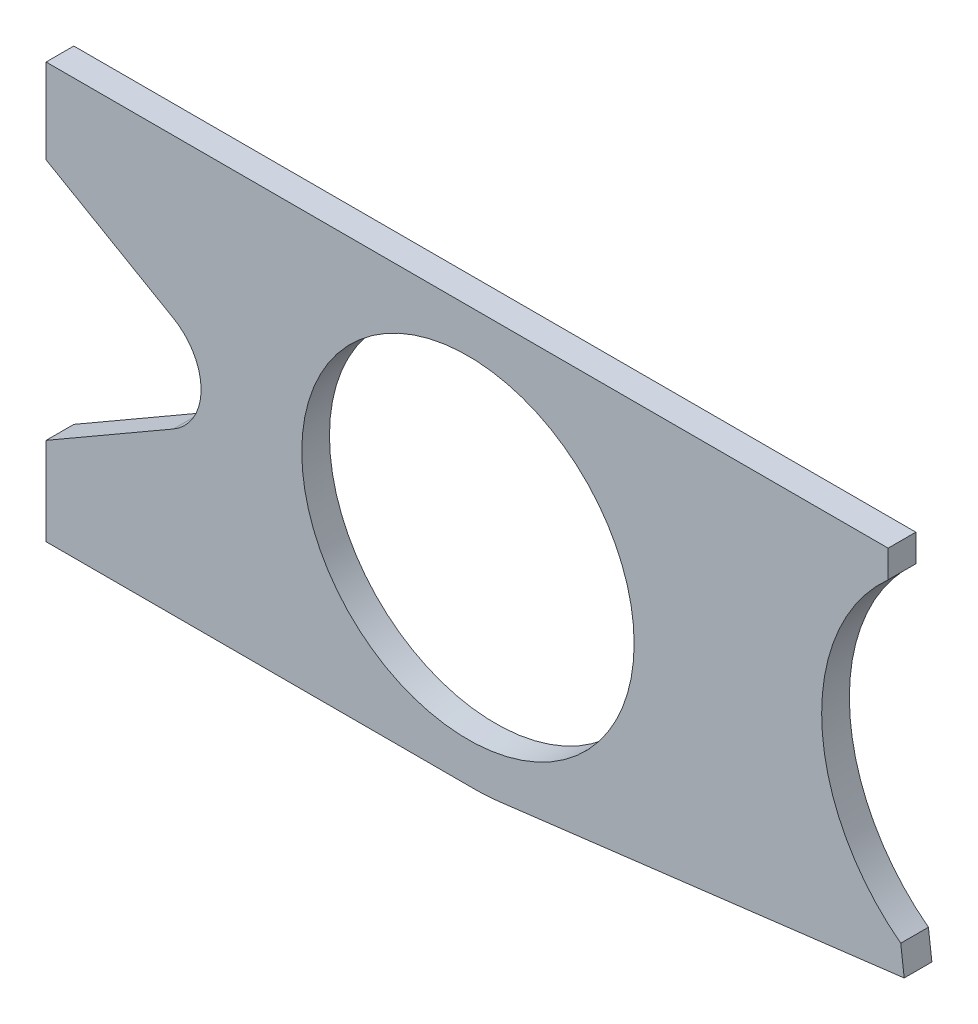
from build123d import *

# Parameters (mm, degrees)
SKETCH1_R           = 60
BOSS_EXTRUDE1_DEPTH = 10


with BuildPart() as part:
    # Sketch1 → Boss-Extrude1 (new body)
    with BuildSketch(Plane.XY):
        with BuildLine():
            Line((-48.3, 63.7), (-48.3, 53.799628252))
            ThreePointArc((-48.3, 53.799628252), (-72.239930825, -2.946590294), (-43.757979913, -57.554575786))
            Line((-43.757979913, -57.554575786), (-42.5, -67.8))
            Line((-42.5, -67.8), (-188.617404673, -85.740961373))
            ThreePointArc((-188.617404673, -85.740961373), (-193.178964964, -86.160109882), (-197.757605429, -86.3))
            Line((-197.757605429, -86.3), (-352.3, -86.3))
            Line((-352.3, -86.3), (-352.3, -54.6))
            Line((-352.3, -54.6), (-306.349572088, -28.070508076))
            ThreePointArc((-306.349572088, -28.070508076), (-296.349572088, -10.75), (-306.349572088, 6.570508076))
            Line((-306.349572088, 6.570508076), (-352.3, 33.1))
            Line((-352.3, 33.1), (-352.3, 63.7))
            Line((-352.3, 63.7), (-48.3, 63.7))
        make_face()
        with Locations((-200, -12)):
            Circle(SKETCH1_R, mode=Mode.SUBTRACT)
    extrude(amount=BOSS_EXTRUDE1_DEPTH)


solid = part.part
